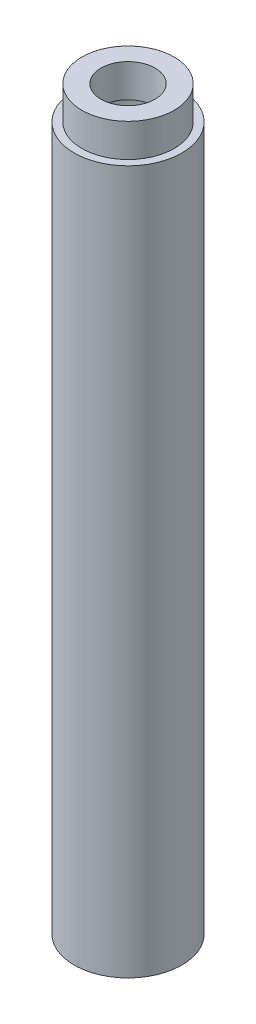
SolidWorks part; units mm, degrees
material "铜"
ref_plane "Front Plane" through (0, 0, 0) normal (0, 0, 1) x (1, 0, 0)
ref_plane "Top Plane" through (0, 0, 0) normal (0, 1, 0) x (1, 0, 0)
ref_plane "Right Plane" through (0, 0, 0) normal (1, 0, 0) x (0, 0, -1)
sketch "Sketch1" plane through (0, 0, 0) normal (0, 0, 1) x (1, 0, 0)
  line L0 (-2.45, 29.9401) -> (-2.45, -2.0599)
  line L1 (-2.35, -2.0599) -> (-2.35, 29.7401)
  line L2 (-2.35, 29.7401) -> (-1.8839, 29.7401)
  line L3 (-1.8839, 29.7401) -> (-1.8839, 29.9401)
  line L4 (-2.1, 29.9401) -> (-2.45, 29.9401)
  line L5 (-2.45, -2.0599) -> (-2.35, -2.0599)
  line L6 (0, -5.4599) -> (0, 34.7467) construction
  line L7 (-2.1, 29.9401) -> (-2.1, 31.447)
  line L8 (-2.1, 31.447) -> (-1.23, 31.447)
  line L9 (-1.23, 31.447) -> (-1.23, 29.9401)
  line L10 (-1.8839, 29.9401) -> (-1.23, 29.9401)
  dimension "D1" = 4.9
  dimension "D2" = 4.7
  dimension "D3" = 4.2
  dimension "D4" = 0.2
  dimension "D5" = 2.46
revolve "Revolve1" add sketch "Sketch1" angle 360 about L6
